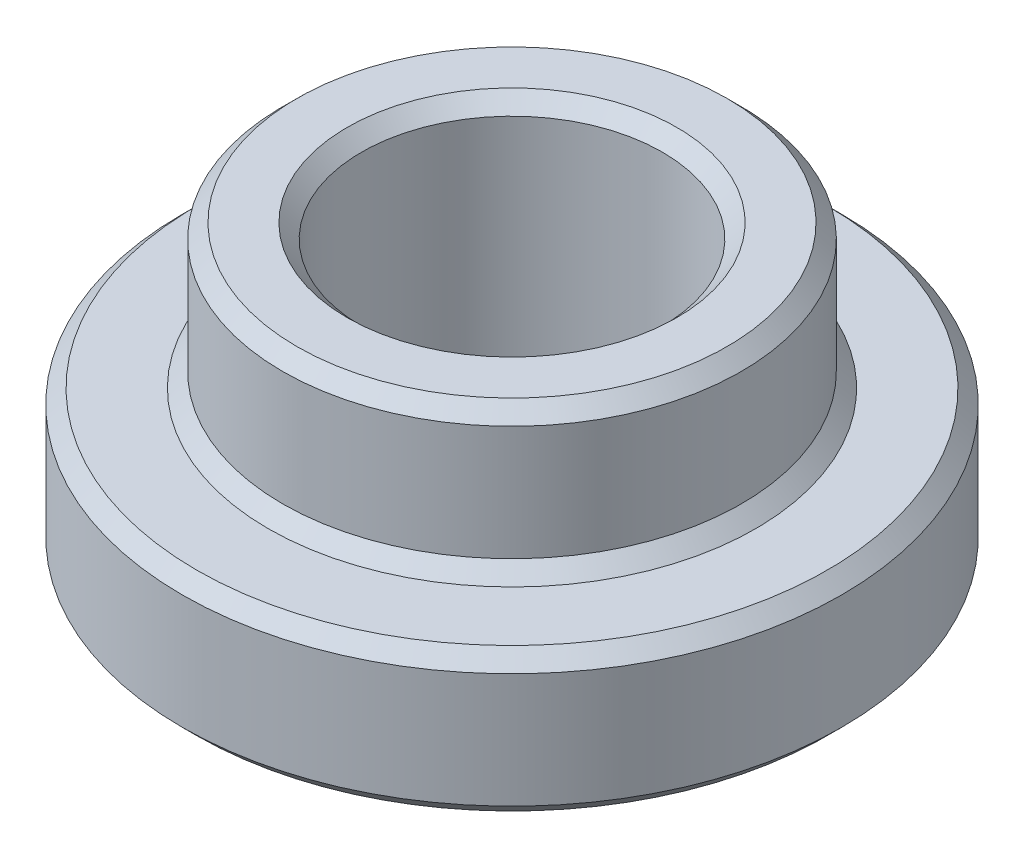
from build123d import *

# Parameters (mm, degrees)
SKETCH1_R           = 23
BOSS_EXTRUDE1_DEPTH = 10
SKETCH2_R           = 16
BOSS_EXTRUDE2_DEPTH = 10
SKETCH3_R           = 10.5
CUT_EXTRUDE1_DEPTH  = 20
CHAMFER1_SIZE       = 1
CHAMFER2_SIZE       = 1


with BuildPart() as part:
    # Sketch1 → Boss-Extrude1 (new body)
    with BuildSketch(Plane(origin=(0, 0, 0), x_dir=(1, 0, 0), z_dir=(0, 1, 0))):
        with Locations(Location((0, 0, 0), (0, 0, 270))):
            Circle(SKETCH1_R)
    extrude(amount=BOSS_EXTRUDE1_DEPTH)

    # Sketch2 → Boss-Extrude2 (add)
    with BuildSketch(Plane(origin=(0, 10, 0), x_dir=(1, 0, 0), z_dir=(0, 1, 0))):
        with Locations(Location((0, 0, 0), (0, 0, 270))):
            Circle(SKETCH2_R)
    extrude(amount=BOSS_EXTRUDE2_DEPTH)

    # Sketch3 → Cut-Extrude1 (cut)
    with BuildSketch(Plane(origin=(0, 20, 0), x_dir=(1, 0, 0), z_dir=(0, 1, 0))):
        with Locations(Location((0, 0, 0), (0, 0, 270))):
            Circle(SKETCH3_R)
    extrude(amount=-CUT_EXTRUDE1_DEPTH, mode=Mode.SUBTRACT)

    # Chamfer1
    chamfer1_edges = [part.edges().sort_by_distance(p)[0] for p in [
        (0, 20, -10.5),
        (0, 0, -23),
        (0, 10, -23),
        (0, 10, -16),
        (0, 20, -16),
    ]]
    chamfer(chamfer1_edges, length=CHAMFER1_SIZE)

    # Chamfer2
    chamfer2_edges = [part.edges().sort_by_distance(p)[0] for p in [
        (0, 0, -10.5),
    ]]
    chamfer(chamfer2_edges, length=CHAMFER2_SIZE)


solid = part.part
